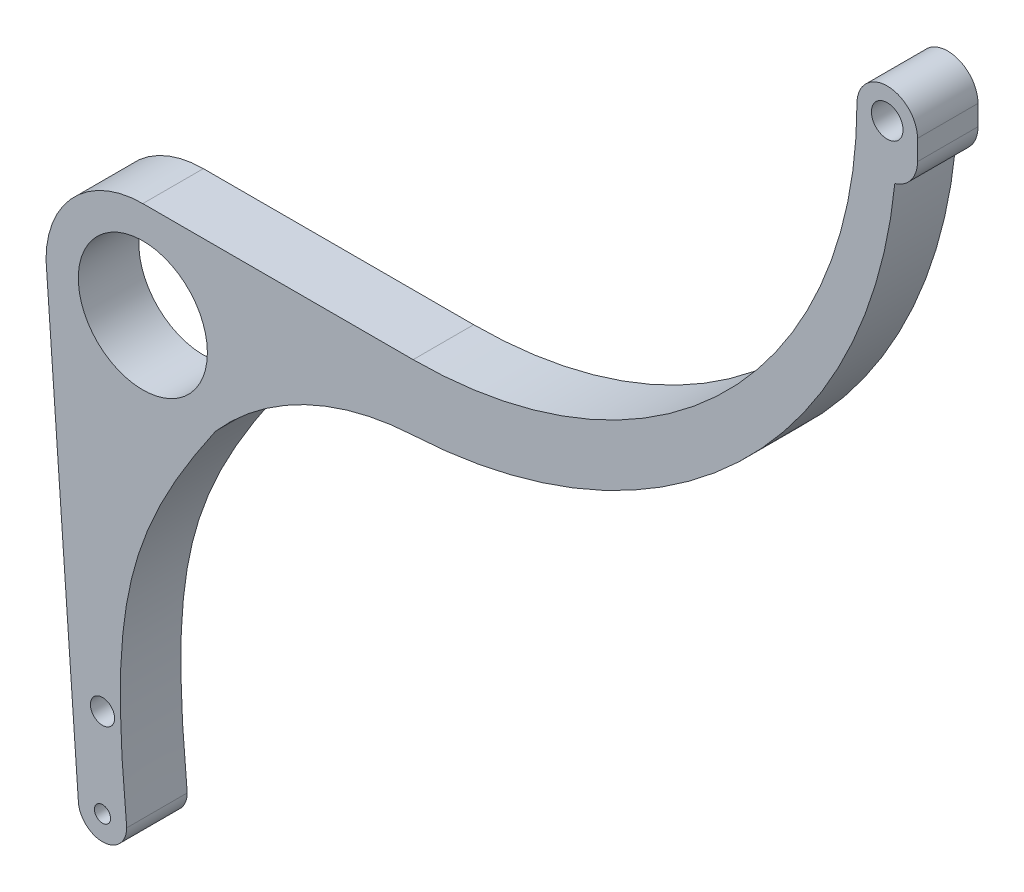
SolidWorks part; units mm, degrees
ref_plane "前视基准面" through (0, 0, 0) normal (0, 0, 1) x (1, 0, 0)
ref_plane "上视基准面" through (0, 0, 0) normal (0, 1, 0) x (1, 0, 0)
ref_plane "右视基准面" through (0, 0, 0) normal (1, 0, 0) x (0, 0, -1)
other "Configuration Table"
sketch "草图1" plane through (0, 0, 0) normal (0, 0, 1) x (1, 0, 0)
  line L0 (-60.8711, 0) -> (72.3657, 0) construction
  line L1 (-84.052, 112) -> (106.5467, 112) construction
  line L2 (0, 22) -> (0, -18.0859) construction
  line L3 (0, -18.0859) -> (10, -18.0859) construction
  line L4 (10, -18.0859) -> (10, 407.7959) construction
  line L5 (-9, 59.8208) -> (-9, -18.0859) construction
  line L6 (-14, 112) -> (-6, 0)
  line L7 (-176.4012, 246) -> (270.3663, 246) construction
  line L8 (77, 485.9134) -> (77, 110.3328) construction
  line L9 (10, 136) -> (77, 136)
  line L10 (187, 246) -> (194.5, 246) construction
  line L11 (202, 246) -> (202, 241)
  line L12 (202, 241) -> (194.1788, 241) construction
  line L13 (70.6056, 267.7759) -> (70.6056, 254.1409) construction
  line L14 (4.2515, 49.8248) -> (157.9856, 49.8248) construction
  line L15 (80.543, 130.5208) -> (80.543, 47.5555) construction
  line L16 (4.7446, 96.1309) -> (49.2871, 96.1309) construction
  line L17 (-29.78, 356) -> (265.8488, 356) construction
  circle A0 centre (0, 0) radius 2
  arc A1 (-6, 0) -> (6, 0) centre (0, 0) ccw
  circle A2 centre (10, 112) radius 16
  arc A3 (10, 136) -> (-14, 112) centre (10, 112) ccw
  circle A4 centre (77, 246) radius 115 construction
  arc A5 (77, 136) -> (187, 246) centre (77, 246) ccw
  arc A6 (202, 246) -> (187, 246) centre (194.5, 246) ccw
  arc A9 (196.3799, 233.4949) -> (202, 241) centre (194.1788, 241) ccw
  arc A10 (77, 119.7674) -> (28.0048, 96.1309) centre (80.543, 49.8248) ccw
  arc A11 (77, 119.7674) -> (196.3799, 233.4949) centre (70.6056, 246) ccw
  circle A12 centre (194.5, 246) radius 3.919
  circle A13 centre (0, 22) radius 3
  spline S0 degree 3 poles (6, 0) (1.5887, 45.6809) (5.6041, 63.6432) (28.0048, 96.1309) knots 0 0 0 0 0.788155 0.788155 0.788155 0.788155
  point P30 (0, 0)
  dimension "D1" = 4
  dimension "D2" = 12
  dimension "D5" = 19
  dimension "D6" = 134
  dimension "D8" = 230
  dimension "D9" = 6.3944
  dimension "D10" = 62.1752
  dimension "D12" = 15.8691
  dimension "D14" = 24
  dimension "D15" = 6
  dimension "D16" = 7.838
  dimension "D17" = 7.5
  dimension "D18" = 220
  dimension "D3" = 112
  dimension "D4" = 9
  dimension "D7" = 67
  dimension "D11" = 70.543
  dimension "D13" = 22
sketch "草图3" plane through (0, 0, 0) normal (0, 0, 1) x (1, 0, 0)
extrude "凸台-拉伸1" add sketch "草图1" along normal blind 15
